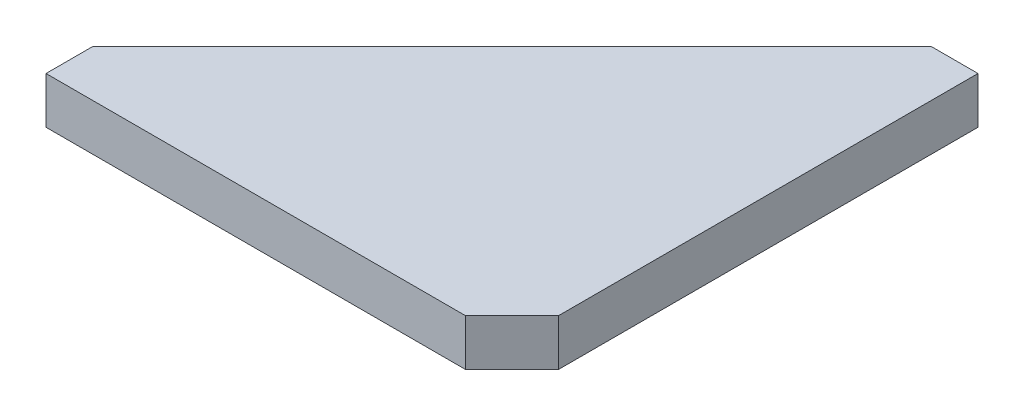
from build123d import *

# Parameters (mm, degrees)
EXTRUDE_1_DEPTH = 20


with BuildPart() as part:
    # 草图1 → 凸台-拉伸1 (new body)
    with BuildSketch(Plane(origin=(0, 0, 0), x_dir=(1, 0, 0), z_dir=(0, 1, 0))):
        Polygon((0, 0), (0, -180), (-20, -200), (-200, -200), (-200, -180), (-20, 0), align=None)
    extrude(amount=EXTRUDE_1_DEPTH)


solid = part.part
